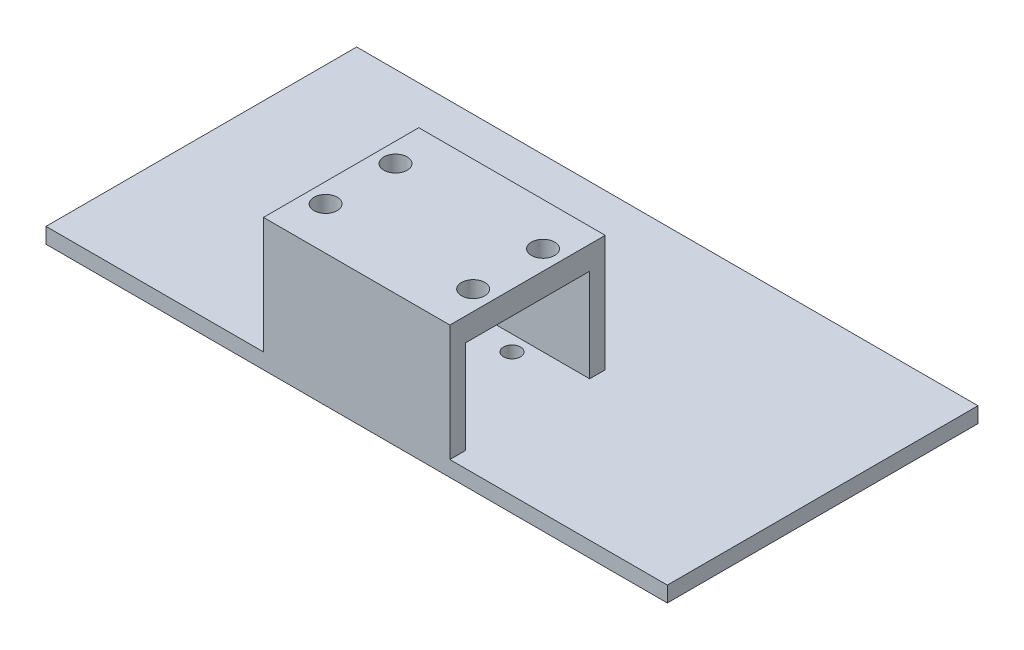
from build123d import *

# Parameters (mm, degrees)
SKETCH1_W           = 80
SKETCH1_H           = 20
SKETCH1_R           = 1.1
BOSS_EXTRUDE1_DEPTH = 2
BOSS_EXTRUDE3_DEPTH = 12
SKETCH4_R           = 1.5
CUT_EXTRUDE1_DEPTH  = 5
SKETCH5_W           = 80
SKETCH5_H           = 2
BOSS_EXTRUDE4_DEPTH = 20


with BuildPart() as part:
    # Sketch1 → Boss-Extrude1 (new body)
    with BuildSketch(Plane(origin=(0, 0, 0), x_dir=(1, 0, 0), z_dir=(0, 1, 0))):
        Rectangle(SKETCH1_W, SKETCH1_H)
        with Locations(Location((-4, 6, 0), (0, 0, 270))):
            Circle(SKETCH1_R, mode=Mode.SUBTRACT)
        with Locations(Location((4, 6, 0), (0, 0, 270))):
            Circle(SKETCH1_R, mode=Mode.SUBTRACT)
        with Locations(Location((-4, -6, 0), (0, 0, 270))):
            Circle(SKETCH1_R, mode=Mode.SUBTRACT)
        with Locations(Location((4, -6, 0), (0, 0, 270))):
            Circle(SKETCH1_R, mode=Mode.SUBTRACT)
    extrude(amount=BOSS_EXTRUDE1_DEPTH)

    # Sketch3 → Boss-Extrude3 (add, symmetric)
    with BuildSketch(Plane(origin=(0, 0, 0), x_dir=(0, 0, -1), z_dir=(1, 0, 0))):
        Polygon((-10, 2), (-8, 2), (-8, 14), (8, 14), (8, 2), (10, 2), (10, 13.782871327), (10, 17), (-10, 17), (-10, 13.782871327), align=None)
    extrude(amount=BOSS_EXTRUDE3_DEPTH, both=True)

    # Sketch4 → Cut-Extrude1 (cut)
    with BuildSketch(Plane(origin=(0, 17, 0), x_dir=(1, 0, 0), z_dir=(0, 1, 0))):
        with Locations(Location((9.5, -4.5, 0), (0, 0, 270))):
            Circle(SKETCH4_R)
        with Locations(Location((-9.5, -4.5, 0), (0, 0, 270))):
            Circle(SKETCH4_R)
        with Locations(Location((-9.5, 4.5, 0), (0, 0, 270))):
            Circle(SKETCH4_R)
        with Locations(Location((9.5, 4.5, 0), (0, 0, 270))):
            Circle(SKETCH4_R)
    extrude(amount=-CUT_EXTRUDE1_DEPTH, mode=Mode.SUBTRACT)

    # Sketch5 → Boss-Extrude4 (add)
    with BuildSketch(Plane.XY.offset(-10)):
        with Locations((0, 1)):
            Rectangle(SKETCH5_W, SKETCH5_H)
    extrude(amount=-BOSS_EXTRUDE4_DEPTH)


solid = part.part
